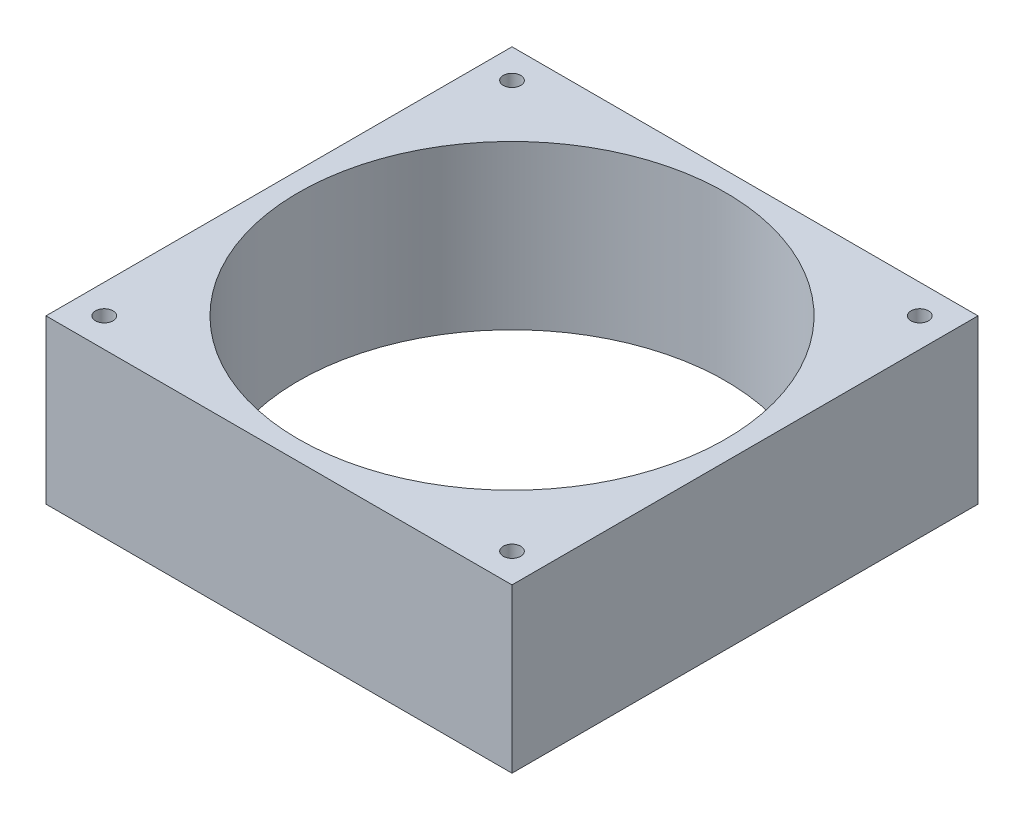
from build123d import *

# Parameters (mm, degrees)
SKETCH_1_W               = 120
SKETCH_1_H               = 120
EXTRUDE_1_DEPTH          = 21
CUT_EXTRUDE_1_DEPTH      = 95.678403028
CUT_EXTRUDE_1_DEPTH_BACK = 95.678403028
SKETCH_2_R               = 55
SKETCH_2_R_2             = 2.25


with BuildPart() as part:
    # 草图1 → 凸台-拉伸1 (new, symmetric)
    with BuildSketch(Plane(origin=(0, 0, 0), x_dir=(1, 0, 0), z_dir=(0, 1, 0))):
        Rectangle(SKETCH_1_W, SKETCH_1_H)
    extrude(amount=EXTRUDE_1_DEPTH, both=True)

    # 草图2 → 切除-拉伸1 (cut, two sides: drawn at the far end of the back side and taken through both)
    with BuildSketch(Plane(origin=(0, 21, 0), x_dir=(1, 0, 0), z_dir=(0, 1, 0)).offset(-CUT_EXTRUDE_1_DEPTH_BACK)):
        with Locations(Location((0, 0, 0), (0, 0, 270))):
            Circle(SKETCH_2_R)
        with Locations(Location((-52.5, 52.5, 0), (0, 0, 270))):
            Circle(SKETCH_2_R_2)
        with Locations(Location((52.5, 52.5, 0), (0, 0, 270))):
            Circle(SKETCH_2_R_2)
        with Locations(Location((52.5, -52.5, 0), (0, 0, 270))):
            Circle(SKETCH_2_R_2)
        with Locations(Location((-52.5, -52.5, 0), (0, 0, 270))):
            Circle(SKETCH_2_R_2)
    extrude(amount=CUT_EXTRUDE_1_DEPTH + CUT_EXTRUDE_1_DEPTH_BACK, mode=Mode.SUBTRACT)


solid = part.part
